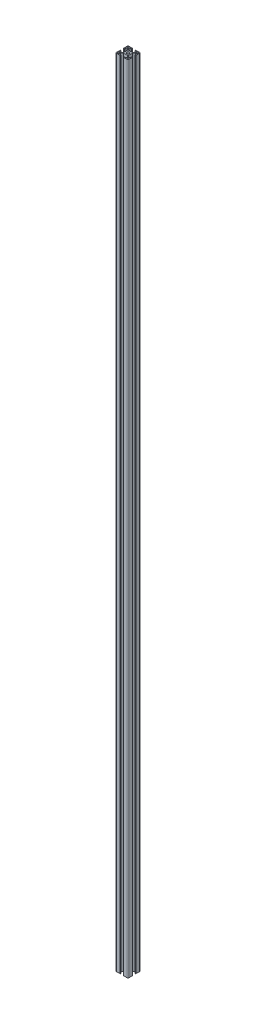
SolidWorks part; units mm, degrees
ref_plane "前视基准面" through (0, 0, 0) normal (0, 0, 1) x (1, 0, 0)
ref_plane "上视基准面" through (0, 0, 0) normal (0, 1, 0) x (1, 0, 0)
ref_plane "右视基准面" through (0, 0, 0) normal (1, 0, 0) x (0, 0, -1)
sketch "草图1" plane through (0, 0, 0) normal (0, 1, 0) x (1, 0, 0)
  line L44 (6.75, -28) -> (11, -28)
  line L45 (11, -28) -> (11, -30)
  line L46 (11, -30) -> (2, -30)
  line L47 (0, -28) -> (0, -19)
  line L48 (0, -19) -> (2, -19)
  line L49 (2, -19) -> (2, -23.25)
  line L50 (28, -30) -> (19, -30)
  line L51 (19, -30) -> (19, -28)
  line L52 (23.25, -28) -> (23.25, -24.6642)
  line L53 (19, -28) -> (23.25, -28)
  line L54 (30, -19) -> (30, -28)
  line L55 (28, -19) -> (30, -19)
  line L56 (28, -23.25) -> (28, -19)
  line L57 (24.6642, -23.25) -> (28, -23.25)
  line L58 (21, -19.5858) -> (24.6642, -23.25)
  line L59 (23.25, -24.6642) -> (19.5858, -21)
  line L60 (6.75, -24.6642) -> (6.75, -28)
  line L61 (2, -23.25) -> (5.3358, -23.25)
  line L62 (5.3358, -23.25) -> (9, -19.5858)
  line L63 (10.4142, -21) -> (6.75, -24.6642)
  line L64 (19.5858, -21) -> (10.4142, -21)
  line L65 (9, -19.5858) -> (9, -10.4142)
  line L66 (21, -10.4142) -> (21, -19.5858)
  line L67 (30, -11) -> (28, -11)
  line L68 (28, -11) -> (28, -6.75)
  line L69 (28, -6.75) -> (24.6642, -6.75)
  line L70 (24.6642, -6.75) -> (21, -10.4142)
  line L71 (19.5858, -9) -> (23.25, -5.3358)
  line L72 (10.4142, -9) -> (19.5858, -9)
  line L73 (6.75, -5.3358) -> (10.4142, -9)
  line L74 (9, -10.4142) -> (5.3358, -6.75)
  line L75 (2, -11) -> (0, -11)
  line L76 (2, -6.75) -> (2, -11)
  line L77 (5.3358, -6.75) -> (2, -6.75)
  line L78 (6.75, -2) -> (6.75, -5.3358)
  line L79 (23.25, -5.3358) -> (23.25, -2)
  line L80 (23.25, -2) -> (19, -2)
  line L81 (19, -2) -> (19, 0)
  line L82 (11, 0) -> (11, -2)
  line L83 (11, -2) -> (6.75, -2)
  line L84 (30, -2) -> (30, -11)
  line L85 (19, 0) -> (28, 0)
  line L86 (2, 0) -> (11, 0)
  line L87 (0, -11) -> (0, -2)
  line L88 (0, -15) -> (30, -15) construction
  line L89 (15, -30) -> (15, 0) construction
  line L90 (0, 0) -> (30, -30) construction
  line L91 (0, -30) -> (30, 0) construction
  arc A9 (0, -28) -> (2, -30) centre (2, -28) ccw
  circle A10 centre (3.375, -26.625) radius 2.1
  circle A11 centre (26.625, -26.625) radius 2.1
  arc A12 (28, -30) -> (30, -28) centre (28, -28) ccw
  circle A13 centre (15, -15) radius 3.4
  circle A14 centre (3.375, -3.375) radius 2.1
  circle A15 centre (26.625, -3.375) radius 2.1
  arc A16 (30, -2) -> (28, 0) centre (28, -2) ccw
  arc A17 (2, 0) -> (0, -2) centre (2, -2) ccw
  dimension "D2" = 15
  dimension "D5" = 6.8
  dimension "D8" = 6
  dimension "D11" = 23.25
  dimension "D12" = 3.375
  dimension "D13" = 23.25
  dimension "D14" = 4.2
  dimension "D15" = 2
  dimension "D16" = 2
  dimension "D23" = 2
  dimension "D24" = 2
  dimension "D1" = 15
  dimension "D3" = 45
  dimension "D4" = 45
  dimension "D6" = 30
  dimension "D7" = 30
  dimension "D9" = 12
  dimension "D10" = 3.375
  dimension "D17" = 11
  dimension "D18" = 8
  dimension "D19" = 2
  dimension "D20" = 2
  dimension "D21" = 11
  dimension "D22" = 8
  dimension "D25" = 2
  dimension "D26" = 2
  dimension "D27" = 6.75
  dimension "D28" = 16.5
  dimension "D29" = 6.75
  dimension "D30" = 16.5
  dimension "D31" = 12
  dimension "D32" = 6
  dimension "D33" = 2
  dimension "D34" = 1
  dimension "D35" = 2
  dimension "D36" = 1
extrude "拉伸1" add sketch "草图1" along normal blind 1940
